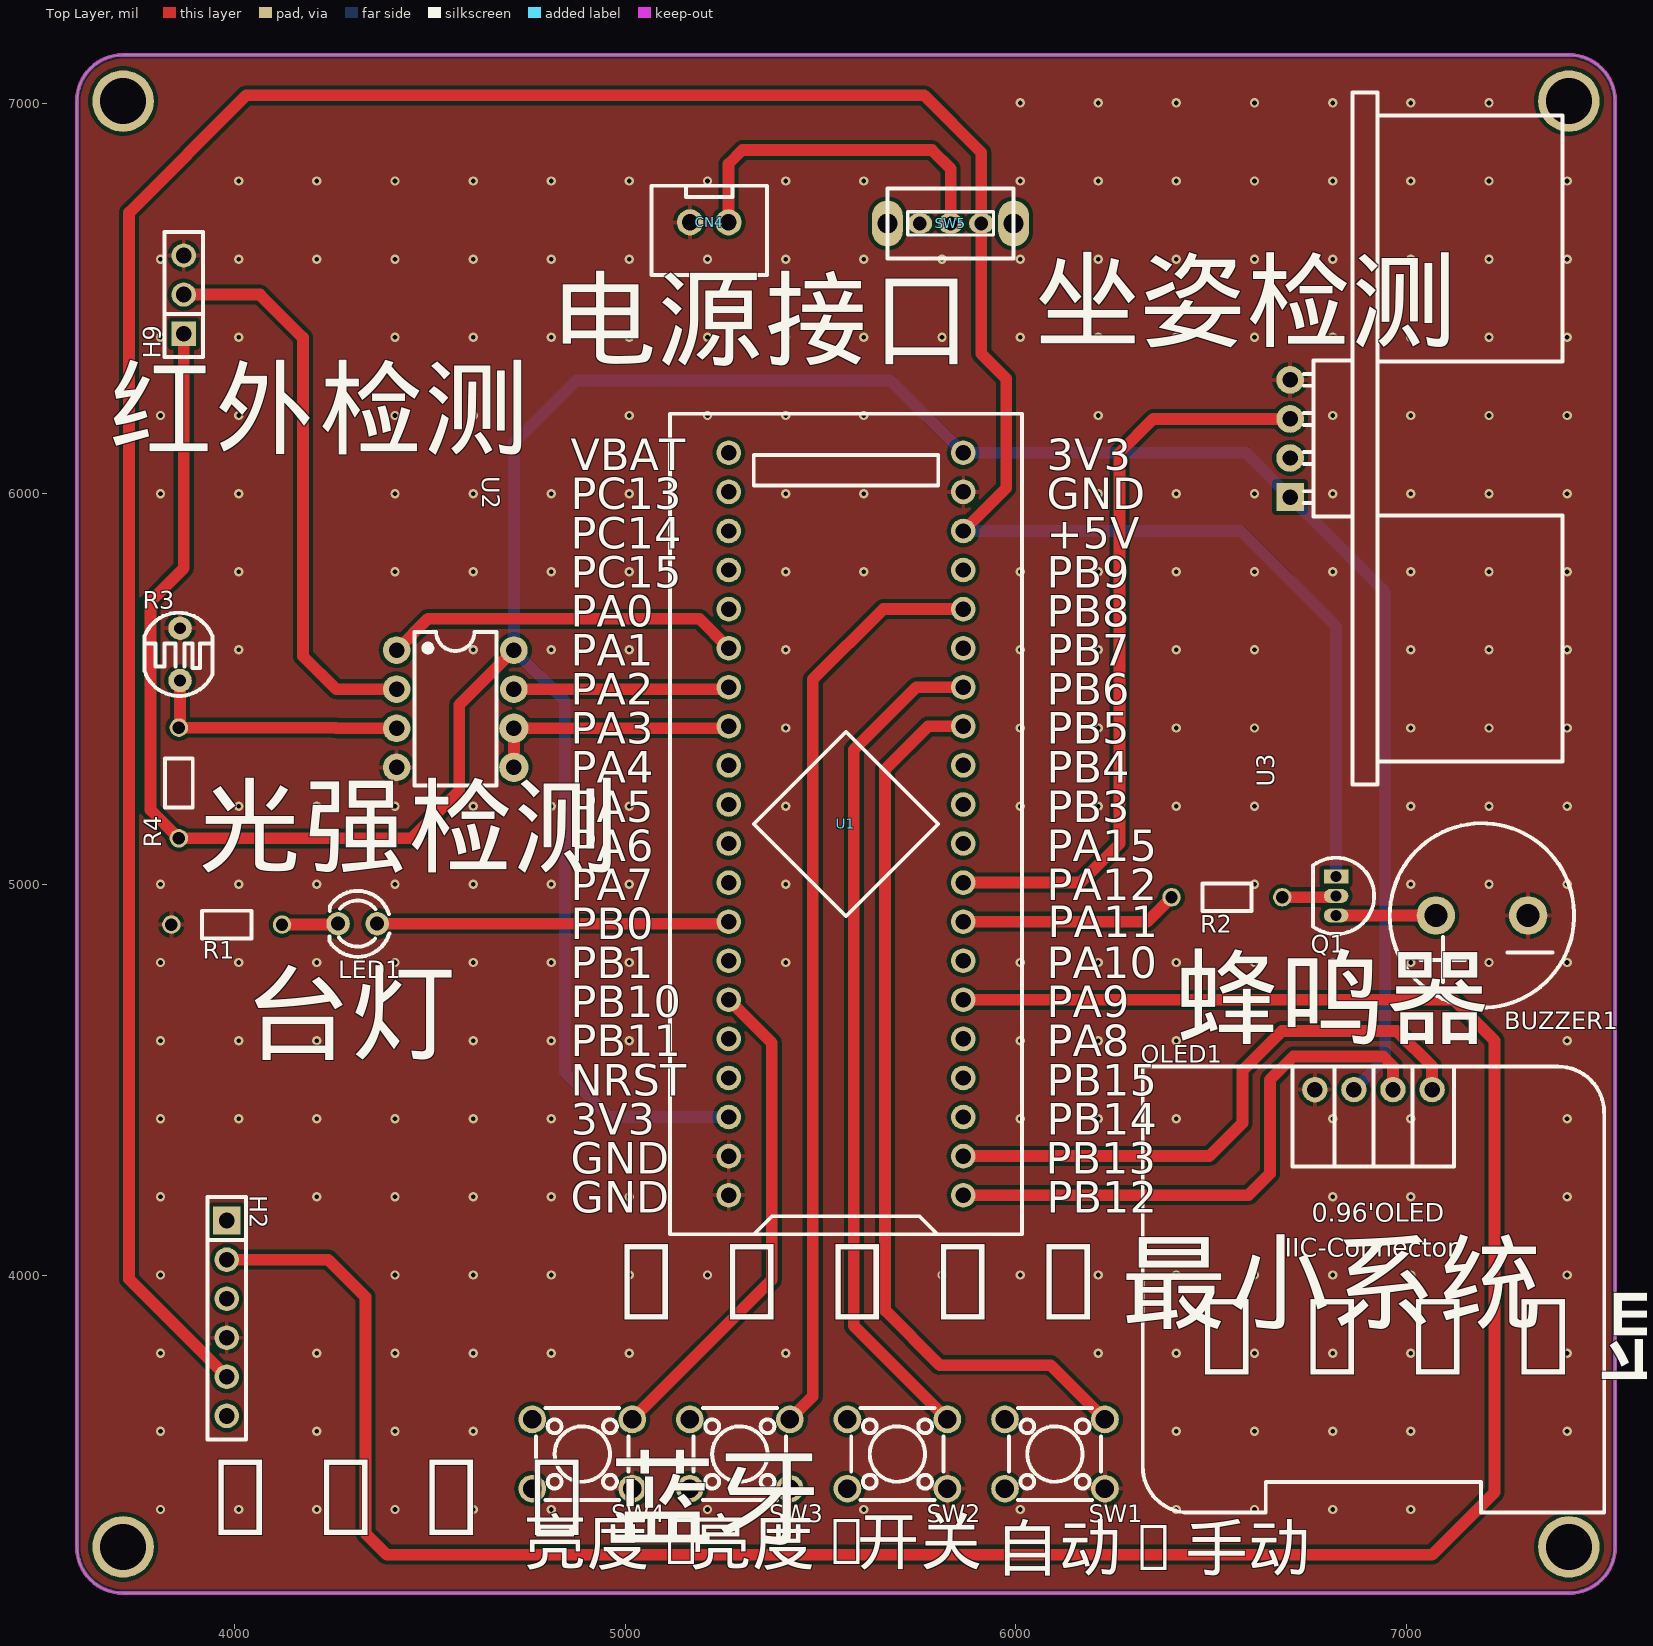
[diagram p0: Top Layer view]
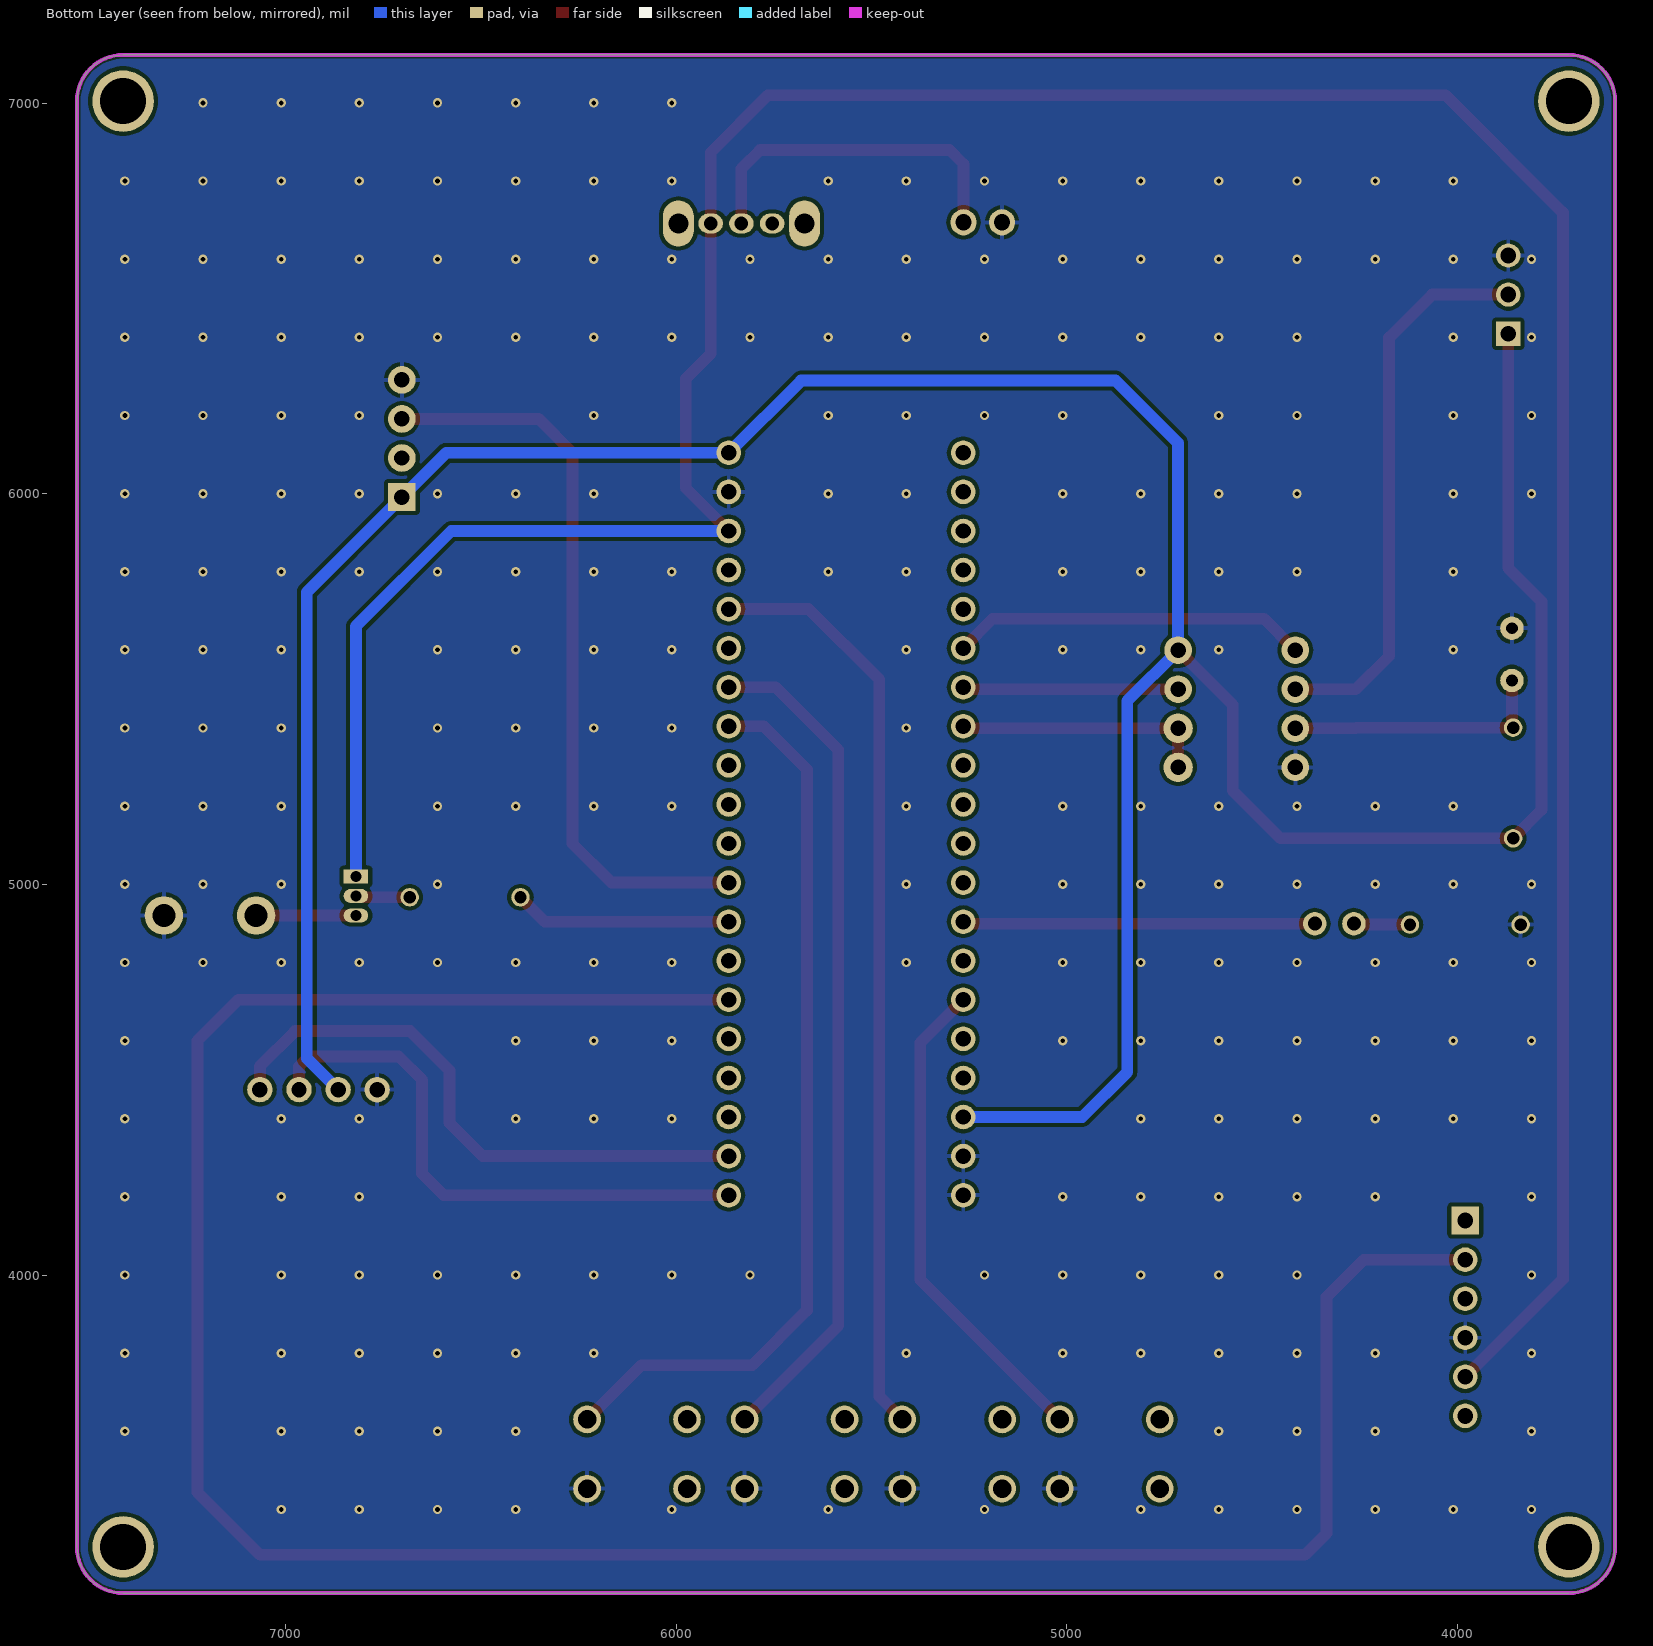
[diagram p1: Bottom Layer view, seen from below]
# Altium PCB MISC51796.pcbdoc
Units mil, origin at the board's own origin, x right, y up, seen from the top; angles counter-clockwise.
Board outline 3937.01 x 3937.01 mil, 2 copper layers (Top Layer, Bottom Layer), stack 62.206 mil thick; 19 components, 44 nets, 107 pads, 247 vias.

## Layer stack, top to bottom
Top Solder Mask Layer: solder mask 0.394, Dk 3.3
Top Layer: signal copper 1.379
Dielectric1: surface 59.449, FR4, Dk 4.5
Bottom Layer: signal copper 1.378
Bottom Solder Mask Layer: solder mask 0.394, Dk 3.3

## Board outline
3714.61,7123.5 ccw(c3714.61,7005.39) 3596.5,7005.39 3596.5,3304.61 ccw(c3714.61,3304.61) 3714.61,3186.5 7415.39,3186.5 ccw(c7415.39,3304.61) 7533.5,3304.61 7533.5,7005.39 ccw(c7415.39,7005.39) 7415.39,7123.5 3714.61,7123.5

## Design rules (kind name [scope] priority, off if disabled: settings)
BoardOutlineClearance copperThickness2oz_1 [All] p2 off: genericclearance=7.99 ignorepadtopadclearanceinfootprint=FALSE except(0: Arc-SplitContinuation Track-SplitContinuation SMDPad-SplitContinuation THPad-SplitContinuation Via-SplitContinuation Fill-SplitContinuation Region-SplitContinuation Poly-SplitContinuation Text-SplitContinuation Hole-SplitContinuation; 5.98: Arc-CutoutEdge Track-CutoutEdge SMDPad-CutoutEdge THPad-CutoutEdge Via-CutoutEdge Text-CutoutEdge; 6.9: Hole-OutlineEdge Hole-CutoutEdge; 10: Poly-OutlineEdge Poly-CutoutEdge; 11.81: Arc-OutlineEdge Track-OutlineEdge SMDPad-OutlineEdge THPad-OutlineEdge Via-OutlineEdge Fill-OutlineEdge Region-OutlineEdge Text-OutlineEdge Fill-CutoutEdge Region-CutoutEdge)
BoardOutlineClearance Plane_innerPlane_1 [All] p4 off: genericclearance=4.02 ignorepadtopadclearanceinfootprint=FALSE except(0: Arc-SplitContinuation Track-SplitContinuation SMDPad-SplitContinuation THPad-SplitContinuation Via-SplitContinuation Fill-SplitContinuation Region-SplitContinuation Poly-SplitContinuation Text-SplitContinuation Hole-SplitContinuation; 5.98: Arc-CutoutEdge Track-CutoutEdge SMDPad-CutoutEdge THPad-CutoutEdge Via-CutoutEdge Text-CutoutEdge; 6.9: Hole-OutlineEdge Hole-CutoutEdge; 10: Poly-OutlineEdge Poly-CutoutEdge; 11.81: Arc-OutlineEdge Track-OutlineEdge SMDPad-OutlineEdge THPad-OutlineEdge Via-OutlineEdge Fill-OutlineEdge Region-OutlineEdge Text-OutlineEdge Fill-CutoutEdge Region-CutoutEdge)
BoardOutlineClearance Copper_copperRegion_1 [All] p6 off: genericclearance=4.02 ignorepadtopadclearanceinfootprint=FALSE except(0: Arc-SplitContinuation Track-SplitContinuation SMDPad-SplitContinuation THPad-SplitContinuation Via-SplitContinuation Fill-SplitContinuation Region-SplitContinuation Poly-SplitContinuation Text-SplitContinuation Hole-SplitContinuation; 5.98: Arc-CutoutEdge Track-CutoutEdge SMDPad-CutoutEdge THPad-CutoutEdge Via-CutoutEdge Text-CutoutEdge; 6.9: Hole-OutlineEdge Hole-CutoutEdge; 10: Poly-OutlineEdge Poly-CutoutEdge; 11.81: Arc-OutlineEdge Track-OutlineEdge SMDPad-OutlineEdge THPad-OutlineEdge Via-OutlineEdge Fill-OutlineEdge Region-OutlineEdge Text-OutlineEdge Fill-CutoutEdge Region-CutoutEdge)
BoardOutlineClearance Copper_copperRegion_copperThickness1oz_1 [All] p8 off: genericclearance=4.02 ignorepadtopadclearanceinfootprint=FALSE except(0: Arc-SplitContinuation Track-SplitContinuation SMDPad-SplitContinuation THPad-SplitContinuation Via-SplitContinuation Fill-SplitContinuation Region-SplitContinuation Poly-SplitContinuation Text-SplitContinuation Hole-SplitContinuation; 5.98: Arc-CutoutEdge Track-CutoutEdge SMDPad-CutoutEdge THPad-CutoutEdge Via-CutoutEdge Text-CutoutEdge; 6.9: Hole-OutlineEdge Hole-CutoutEdge; 10: Poly-OutlineEdge Poly-CutoutEdge; 11.81: Arc-OutlineEdge Track-OutlineEdge SMDPad-OutlineEdge THPad-OutlineEdge Via-OutlineEdge Fill-OutlineEdge Region-OutlineEdge Text-OutlineEdge Fill-CutoutEdge Region-CutoutEdge)
BoardOutlineClearance Copper_copperRegion_Copper_copperRegion_1 [All] p10 off: genericclearance=4.02 ignorepadtopadclearanceinfootprint=FALSE except(0: Arc-SplitContinuation Track-SplitContinuation SMDPad-SplitContinuation THPad-SplitContinuation Via-SplitContinuation Fill-SplitContinuation Region-SplitContinuation Poly-SplitContinuation Text-SplitContinuation Hole-SplitContinuation; 5.98: Arc-CutoutEdge Track-CutoutEdge SMDPad-CutoutEdge THPad-CutoutEdge Via-CutoutEdge Text-CutoutEdge; 6.9: Hole-OutlineEdge Hole-CutoutEdge; 10: Poly-OutlineEdge Poly-CutoutEdge; 11.81: Arc-OutlineEdge Track-OutlineEdge SMDPad-OutlineEdge THPad-OutlineEdge Via-OutlineEdge Fill-OutlineEdge Region-OutlineEdge Text-OutlineEdge Fill-CutoutEdge Region-CutoutEdge)
BoardOutlineClearance copperThickness1oz_1 [All] p12: genericclearance=4.02 ignorepadtopadclearanceinfootprint=FALSE except(0: Arc-SplitContinuation Track-SplitContinuation SMDPad-SplitContinuation THPad-SplitContinuation Via-SplitContinuation Fill-SplitContinuation Region-SplitContinuation Poly-SplitContinuation Text-SplitContinuation Hole-SplitContinuation; 5.98: Arc-CutoutEdge Track-CutoutEdge SMDPad-CutoutEdge THPad-CutoutEdge Via-CutoutEdge Text-CutoutEdge; 6.9: Hole-OutlineEdge Hole-CutoutEdge; 10: Poly-OutlineEdge Poly-CutoutEdge; 11.81: Arc-OutlineEdge Track-OutlineEdge SMDPad-OutlineEdge THPad-OutlineEdge Via-OutlineEdge Fill-OutlineEdge Region-OutlineEdge Text-OutlineEdge Fill-CutoutEdge Region-CutoutEdge)
Clearance copperThickness2oz [All] p1 off: gap=7.99 ignorepadtopadclearanceinfootprint=FALSE except(5.98: SMDPad-Track SMDPad-SMDPad THPad-Track SMDPad-THPad THPad-THPad Track-Via SMDPad-Via THPad-Via Via-Via Fill-SMDPad Region-SMDPad Fill-THPad Region-THPad Fill-Via Region-Via Fill-Fill Fill-Region Region-Region Arc-Track Arc-SMDPad Arc-THPad Arc-Via Fill-Arc Region-Arc Arc-Arc Text-Track SMDPad-Text Text-THPad Text-Via Fill-Text Region-Text Arc-Text Text-Text; 6.9: Hole-Track Hole-SMDPad Hole-THPad Hole-Via Fill-Hole Region-Hole Hole-Arc Hole-Text; 10: Poly-Track Poly-SMDPad Poly-THPad Poly-Via Poly-Fill Poly-Region Poly-Poly Poly-Arc Poly-Text Poly-Hole; 11.81: Fill-Track Region-Track)
Clearance Plane_innerPlane [All] p3 off: gap=4.02 ignorepadtopadclearanceinfootprint=FALSE except(5.98: SMDPad-Track SMDPad-SMDPad THPad-Track SMDPad-THPad THPad-THPad Track-Via SMDPad-Via THPad-Via Via-Via Fill-SMDPad Region-SMDPad Fill-THPad Region-THPad Fill-Via Region-Via Fill-Fill Fill-Region Region-Region Arc-Track Arc-SMDPad Arc-THPad Arc-Via Fill-Arc Region-Arc Arc-Arc Text-Track SMDPad-Text Text-THPad Text-Via Fill-Text Region-Text Arc-Text Text-Text; 6.9: Hole-Track Hole-SMDPad Hole-THPad Hole-Via Fill-Hole Region-Hole Hole-Arc Hole-Text; 10: Poly-Track Poly-SMDPad Poly-THPad Poly-Via Poly-Fill Poly-Region Poly-Poly Poly-Arc Poly-Text Poly-Hole; 11.81: Fill-Track Region-Track)
Clearance Copper_copperRegion [All] p5 off: gap=4.02 ignorepadtopadclearanceinfootprint=FALSE except(5.98: SMDPad-Track SMDPad-SMDPad THPad-Track SMDPad-THPad THPad-THPad Track-Via SMDPad-Via THPad-Via Via-Via Fill-SMDPad Region-SMDPad Fill-THPad Region-THPad Fill-Via Region-Via Fill-Fill Fill-Region Region-Region Arc-Track Arc-SMDPad Arc-THPad Arc-Via Fill-Arc Region-Arc Arc-Arc Text-Track SMDPad-Text Text-THPad Text-Via Fill-Text Region-Text Arc-Text Text-Text; 6.9: Hole-Track Hole-SMDPad Hole-THPad Hole-Via Fill-Hole Region-Hole Hole-Arc Hole-Text; 10: Poly-Track Poly-SMDPad Poly-THPad Poly-Via Poly-Fill Poly-Region Poly-Poly Poly-Arc Poly-Text Poly-Hole; 11.81: Fill-Track Region-Track)
Clearance Copper_copperRegion_copperThickness1oz [All] p7 off: gap=4.02 ignorepadtopadclearanceinfootprint=FALSE except(5.98: SMDPad-Track SMDPad-SMDPad THPad-Track SMDPad-THPad THPad-THPad Track-Via SMDPad-Via THPad-Via Via-Via Fill-SMDPad Region-SMDPad Fill-THPad Region-THPad Fill-Via Region-Via Fill-Fill Fill-Region Region-Region Arc-Track Arc-SMDPad Arc-THPad Arc-Via Fill-Arc Region-Arc Arc-Arc Text-Track SMDPad-Text Text-THPad Text-Via Fill-Text Region-Text Arc-Text Text-Text; 6.9: Hole-Track Hole-SMDPad Hole-THPad Hole-Via Fill-Hole Region-Hole Hole-Arc Hole-Text; 10: Poly-Track Poly-SMDPad Poly-THPad Poly-Via Poly-Fill Poly-Region Poly-Poly Poly-Arc Poly-Text Poly-Hole; 11.81: Fill-Track Region-Track)
Clearance Copper_copperRegion_Copper_copperRegion [All] p9 off: gap=4.02 ignorepadtopadclearanceinfootprint=FALSE except(5.98: SMDPad-Track SMDPad-SMDPad THPad-Track SMDPad-THPad THPad-THPad Track-Via SMDPad-Via THPad-Via Via-Via Fill-SMDPad Region-SMDPad Fill-THPad Region-THPad Fill-Via Region-Via Fill-Fill Fill-Region Region-Region Arc-Track Arc-SMDPad Arc-THPad Arc-Via Fill-Arc Region-Arc Arc-Arc Text-Track SMDPad-Text Text-THPad Text-Via Fill-Text Region-Text Arc-Text Text-Text; 6.9: Hole-Track Hole-SMDPad Hole-THPad Hole-Via Fill-Hole Region-Hole Hole-Arc Hole-Text; 10: Poly-Track Poly-SMDPad Poly-THPad Poly-Via Poly-Fill Poly-Region Poly-Poly Poly-Arc Poly-Text Poly-Hole; 11.81: Fill-Track Region-Track)
Clearance copperThickness1oz [All] p11: gap=4.02 ignorepadtopadclearanceinfootprint=FALSE except(5.98: SMDPad-Track SMDPad-SMDPad THPad-Track SMDPad-THPad THPad-THPad Track-Via SMDPad-Via THPad-Via Via-Via Fill-SMDPad Region-SMDPad Fill-THPad Region-THPad Fill-Via Region-Via Fill-Fill Fill-Region Region-Region Arc-Track Arc-SMDPad Arc-THPad Arc-Via Fill-Arc Region-Arc Arc-Arc Text-Track SMDPad-Text Text-THPad Text-Via Fill-Text Region-Text Arc-Text Text-Text; 6.9: Hole-Track Hole-SMDPad Hole-THPad Hole-Via Fill-Hole Region-Hole Hole-Arc Hole-Text; 10: Poly-Track Poly-SMDPad Poly-THPad Poly-Via Poly-Fill Poly-Region Poly-Poly Poly-Arc Poly-Text Poly-Hole; 11.81: Fill-Track Region-Track)
DiffPairsRouting differentialPair [All] p1: maxlimit=6 minlimit=6 mostfreqgap=6 toplayer_minwidth=5 toplayer_prefwidth=10 toplayer_maxwidth=100 toplayer_mingap=6 toplayer_prefgap=6 toplayer_maxgap=6 bottomlayer_minwidth=5 bottomlayer_prefwidth=10 bottomlayer_maxwidth=100 bottomlayer_mingap=6 bottomlayer_prefgap=6 bottomlayer_maxgap=6 maxuncoupledlength=10
HoleToHoleClearance otherClearance [All] p1: gap=11.81 allowstackedmicrovias=TRUE
Length netLength [All] p1: minlimit=0 maxlimit=0
PasteMaskExpansion pasteMaskExpansion [All] p1: expansion=0
PlaneConnect innerPlane [All] p1: planeconnectstyle=Relief reliefexpansion=20 reliefentries=4 reliefconductorwidth=10 reliefairgap=10
PolygonConnect copperRegion_copperThickness1oz [All] p1 off: connectstyle=Relief reliefconductorwidth=10 reliefentries=4 polygonreliefangle="90 Angle" airgapwidth=10 via.connectstyle=Relief via.reliefconductorwidth=10 via.reliefentries=4 via.polygonreliefangle="90 Angle" via.airgapwidth=10
PolygonConnect copperRegion_Copper_copperRegion [All] p2 off: connectstyle=Relief reliefconductorwidth=10 reliefentries=4 polygonreliefangle="90 Angle" airgapwidth=10 via.connectstyle=Relief via.reliefconductorwidth=10 via.reliefentries=4 via.polygonreliefangle="90 Angle" via.airgapwidth=10
PolygonConnect copperRegion [All] p3: connectstyle=Relief reliefconductorwidth=10 reliefentries=4 polygonreliefangle="90 Angle" airgapwidth=10 via.connectstyle=Relief via.reliefconductorwidth=10 via.reliefentries=4 via.polygonreliefangle="90 Angle" via.airgapwidth=10
RoutingVias viaSize [All] p1: holewidth=12.01 width=24.02 viastyle="Through Hole" minholewidth=11.81 minwidth=19.68 maxholewidth=248.03 maxwidth=393.7
SolderMaskExpansion solderMaskExpansion [IsVia] p1: expansion=-1000 istentingtop=TRUE
SolderMaskExpansion solderMaskExpansion [All] p2: expansion=2 istentingtop=FALSE
Width copperThickness2oz_2 [All] p1 off: maxlimit=100 minlimit=8 preferedwidth=10
Width copperThickness1oz_2 [All] p2: maxlimit=100 minlimit=5 preferedwidth=10

## Components (designator, comment, footprint, x,y, rotation, side; value= is the part's Value field where it differs from the comment)
BUZZER1 "buzzer" BUZ-TH_BD12.0-P6.00-D0.9-RD 7192.78,4920.87 r180 top
CN4 "XH2.54*2P_直插" CONN-TH_2P-P2.50-XH2.54-2P 5215,6695 r0 top
H2 "" HDR-TH_6P-P2.54-V-F 3980,3890 r270 top
H9 "" HDR-TH_3P-P2.54-V-F 3870,6510 r90 top
LED1 "" LED_TH-3mm 4314.99,4899.94 r180 top
OLED1 "" 0.96OLED_4P 6915,4475 r0 top
Q1 "" S8550P_TO-92 6819.29,4970.87 r270 top
R1 "100" Res_1/8W 3980,4900 r180 top
R2 "1kΩ" Res_1/8W 6540,4970 r180 top
R3 "GL5549(80-100)" RES-TH_L5.1-W4.3-P3.40-D0.5 3860.5,5589.21 r0 top
R4 "10kΩ" Res_1/8W 3860,5260 r90 top
SW1 "" SW-TH_4P-L6.0-W6.0-P4.50-LS6.5 6099.85,3542.47 r180 top
SW2 "" SW-TH_4P-L6.0-W6.0-P4.50-LS6.5 5696.57,3542.47 r180 top
SW3 "" SW-TH_4P-L6.0-W6.0-P4.50-LS6.5 5293.28,3542.47 r180 top
SW4 "" SW-TH_4P-L6.0-W6.0-P4.50-LS6.5 4890,3542.47 r180 top
SW5 "" 拨动开关 5837.9,6692.05 r180 top
U1 "STM32F103C8T6-Card" CONN-TH_L53.3-W22.9_STM32F103C8T6-CARD 5565,5155 r90 top
U2 "ADC0832BCN" PDIP-8_L9.6-W6.4-P2.54-LS7.6-BL 4565,5450 r270 top
U3 "HC-SR04" TH_HC-SR04V 6701.72,6141.72 r90 top

## Footprints (in the part's own frame and the unit in brackets; to place one, negate y for a bottom-side part, rotate by r counter-clockwise, add the part's x,y. Pads: shape width x height; smd on the part's side, far side on the other; paste and mask are expansions set on the pad)
0.96OLED_4P [mm]
  round 1.65 hole 1 copper offset 0,0: 1(-3.81,-0.001) 2(-1.27,0.002) 3(1.27,0.002) 4(3.81,0.002)
  silkscreen extent -15,-27.5 15,1.5
BUZ-TH_BD12.0-P6.00-D0.9-RD [mm]
  round 2.5 hole 1.5 paste+0 mask+0.05: 1(-3,0) 2(3,0)
  silkscreen extent -5.99,-5.99 5.99,5.99
CONN-TH_2P-P2.50-XH2.54-2P [mm]
  round 1.7 hole 1.05 paste+0 mask+0.05: 1(1.25,0) 2(-1.25,0)
  silkscreen extent -3.75,-3.42 3.75,2.37
CONN-TH_L53.3-W22.9_STM32F103C8T6-CARD [mm]
  round 1.6 hole 1: 1(-24.13,-7.62) 2(-21.59,-7.62) 3(-19.05,-7.62) 4(-16.51,-7.62) 5(-13.97,-7.62) 6(-11.43,-7.62) 7(-8.89,-7.62) 8(-6.35,-7.62) 9(-3.81,-7.62) 10(-1.27,-7.62) 11(1.27,-7.62) 12(3.81,-7.62) 13(6.35,-7.62) 14(8.89,-7.62) 15(11.43,-7.62) 16(13.97,-7.62) 17(16.51,-7.62) 18(19.05,-7.62) 19(21.59,-7.62) 20(24.13,-7.62) 21(24.13,7.62) 22(21.59,7.62) 23(19.05,7.62) 24(16.51,7.62) 25(13.97,7.62) 26(11.43,7.62) 27(8.89,7.62) 28(6.35,7.62) 29(3.81,7.62) 30(1.27,7.62) 31(-1.27,7.62) 32(-3.81,7.62) 33(-6.35,7.62) 34(-8.89,7.62) 35(-11.43,7.62) 36(-13.97,7.62) 37(-16.51,7.62) 38(-19.05,7.62) 39(-21.59,7.62) 40(-24.13,7.62)
  silkscreen extent -26.67,-11.43 26.67,11.43
HDR-TH_3P-P2.54-V-F [mil]
  rect 62x62 hole 40.16: 1(-100,0)
  round 62 hole 40.16: 2(0,0) 3(100,0)
  silkscreen extent -160,-49 160,49
HDR-TH_6P-P2.54-V-F [mm]
  rect 1.8x1.8 hole 1.02: 1(-6.35,0)
  round 1.6 hole 1.02: 2(-3.81,0) 3(-1.27,0) 4(1.27,0) 5(3.81,0) 6(6.35,0)
  silkscreen extent -7.87,-1.25 7.87,1.25
LED_TH-3mm [mil]
  round 60 hole 36 paste+0 mask+2: 1(-50,0) 2(50,0)
  silkscreen extent -81,-84 72,85
PDIP-8_L9.6-W6.4-P2.54-LS7.6-BL [mm]
  round 1.8 hole 1: 1(-3.81,-3.81) 2(-1.27,-3.81) 3(1.27,-3.81) 4(3.81,-3.81) 7(-1.27,3.81) 8(-3.81,3.81)
  round 1.905 hole 1: 5(3.81,3.81) 6(1.27,3.81)
  silkscreen extent -5,-2.64 5,2.67
RES-TH_L5.1-W4.3-P3.40-D0.5 [mil]
  round 60 hole 30: 1(0,66.93) 2(0,-66.93)
  silkscreen extent -91,-106 83,106
Res_1/8W [mil]
  round 47.2 hole 31.5 paste+0 mask+2: 1(-141.7,2.48) 2(141.7,2.48)
  silkscreen extent -63,-33 63,38
S8550P_TO-92 [mm]
  rect 0.9x1.6 hole 0.7 paste+0 mask+0.051: 1(-1.27,0)
  oval 0.9x1.6 hole 0.7 paste+0 mask+0.051: 2(0,0) 3(1.27,0)
  silkscreen extent -2.48,-1.5 2.48,2.48
SW-TH_4P-L6.0-W6.0-P4.50-LS6.5 [mm]
  round 1.8 hole 1.2: 1(-3.25,2.25) 2(3.25,2.25) 3(-3.25,-2.25) 4(3.25,-2.25)
  silkscreen extent -3,-3 3,3
TH_HC-SR04V [mm]
  rect 1.8x1.8 hole 1.001: 1(-3.81,0)
  round 1.8 hole 1.001: 2(-1.27,0) 3(1.27,0) 4(3.81,0)
  silkscreen extent -22.5,-17.7 22.5,-0.89
拨动开关 [mil]
  oval 63x51.2 hole 35.4 paste+0 mask+2: 1(-73.4,0) 2(5,0) 3(84,0)
  oval 78.7x118.1 hole 51.2 paste+0 mask+2: 4(166.7,0) 5(-156.1,0)
  silkscreen extent -156,-90 167,90

## Free pads (board coordinates)
  round 157.48 hole 118.11: 1(3714.61,7005.39) 1(3714.61,3304.61) 1(7415.39,7005.39) 1(7415.39,3304.61)

## Via types
v1: diameter 24.02, hole 12, Top Layer to Bottom Layer, 247 vias

## Nets (pads, with @x,y where several pads share a name; then routed paths per layer and width w, separated by ;. In a path a pad name is that pad's centre, name@x,y a point inside that pad or via, vN(x,y) a via of type N, cw(c..) or ccw(c..) an arc to the next point about the centre after c; other vN are vias at no path point)
$1N17118: CN4.1 SW5.2 | length 892.6
  Top Layer w30: CN4.1 5264.22,6844.22 5300,6880 5785,6880 5832.9,6832.1 SW5.2
$1N17160: LED1.2 R1.1 | length 144.3
  Top Layer w30: R1.1 4262.57,4897.52 LED1.2
$1N17185: BUZZER1.2 Q1.3 | length 255.4
  Top Layer w30: Q1.3 BUZZER1.2
$1N17199: Q1.2 R2.1 | length 139
  Top Layer w30: R2.1 6815.95,4967.52 Q1.2
+5V: H2.5 Q1.1 SW5.1 U1.18 | length 8185.7
  Top Layer w30: H2.5 3730,3990 3730,6720 4030,7020 5765,7020 5911.3,6873.7 SW5.1 5911.3,6358.7 5975,6295 5975,6015 U1.18
  Bottom Layer w30: U1.18 6575,5905 6819.29,5660.71 Q1.1
CH0: H9.2 U2.2 | length 1440.8
  Top Layer w30: H9.2 4065,6510 4175,6400 4175,5585 4260,5500 U2.2
CH1: R3.2 R4.2 U2.3 | length 680
  Top Layer w30: R3.2 3860.5,5404.68 R4.2 4258.3,5401.7 4260,5400 U2.3
GND: BUZZER1.1 CN4.2 H2.4 H9.3 OLED1.1 R1.2 R3.1 SW1.1 SW2.1 SW3.1 SW4.1 U1.19 U1.39 U1.40 U2.4 U3.4
  other v1: 3810.6,3400.6 4010.6,3400.6 4210.6,3400.6 4410.6,3400.6 4610.6,3400.6 4810.6,3400.6 5210.6,3400.6 5610.6,3400.6 6010.6,3400.6 6410.6,3400.6 6610.6,3400.6 6810.6,3400.6 7010.6,3400.6 3810.6,3600.6 4210.6,3600.6 4410.6,3600.6 4610.6,3600.6 6410.6,3600.6 6610.6,3600.6 6810.6,3600.6 7010.6,3600.6 7410.6,3600.6 3810.6,3800.6 4210.6,3800.6 4410.6,3800.6 4610.6,3800.6 4810.6,3800.6 5010.6,3800.6 5410.6,3800.6 6210.6,3800.6 6410.6,3800.6 6610.6,3800.6 6810.6,3800.6 7010.6,3800.6 7410.6,3800.6 3810.6,4000.6 4410.6,4000.6 4610.6,4000.6 4810.6,4000.6 5010.6,4000.6 5210.6,4000.6 5810.6,4000.6 6010.6,4000.6 6210.6,4000.6 6410.6,4000.6 6610.6,4000.6 6810.6,4000.6 7010.6,4000.6 7410.6,4000.6 3810.6,4200.6 4210.6,4200.6 4410.6,4200.6 4610.6,4200.6 4810.6,4200.6 5010.6,4200.6 6810.6,4200.6 7010.6,4200.6 7410.6,4200.6 3810.6,4400.6 4010.6,4400.6 4210.6,4400.6 4410.6,4400.6 4610.6,4400.6 4810.6,4400.6 6010.6,4400.6 6210.6,4400.6 6410.6,4400.6 6810.6,4400.6 7010.6,4400.6 7410.6,4400.6 3810.6,4600.6 4010.6,4600.6 4210.6,4600.6 4410.6,4600.6 4610.6,4600.6 4810.6,4600.6 5010.6,4600.6 6010.6,4600.6 6210.6,4600.6 6410.6,4600.6 7410.6,4600.6 3810.6,4800.6 4010.6,4800.6 4210.6,4800.6 4410.6,4800.6 4610.6,4800.6 4810.6,4800.6 5010.6,4800.6 5410.6,4800.6 6010.6,4800.6 6210.6,4800.6 6410.6,4800.6 6610.6,4800.6 6810.6,4800.6 7010.6,4800.6 7210.6,4800.6 7410.6,4800.6 3810.6,5000.6 4010.6,5000.6 4210.6,5000.6 4410.6,5000.6 4610.6,5000.6 4810.6,5000.6 5010.6,5000.6 5410.6,5000.6 6610.6,5000.6 7010.6,5000.6 7210.6,5000.6 7410.6,5000.6 4010.6,5200.6 4210.6,5200.6 4410.6,5200.6 4610.6,5200.6 4810.6,5200.6 5010.6,5200.6 5410.6,5200.6 6010.6,5200.6 6210.6,5200.6 6410.6,5200.6 6610.6,5200.6 7010.6,5200.6 7210.6,5200.6 7410.6,5200.6 5410.6,5400.6 6010.6,5400.6 6210.6,5400.6 6410.6,5400.6 6610.6,5400.6 7010.6,5400.6 7210.6,5400.6 7410.6,5400.6 4010.6,5600.6 4610.6,5600.6 4810.6,5600.6 5010.6,5600.6 5410.6,5600.6 6010.6,5600.6 6210.6,5600.6 6410.6,5600.6 6610.6,5600.6 7010.6,5600.6 7210.6,5600.6 7410.6,5600.6 4010.6,5800.6 4410.6,5800.6 4610.6,5800.6 4810.6,5800.6 5010.6,5800.6 5410.6,5800.6 5610.6,5800.6 6010.6,5800.6 6210.6,5800.6 6410.6,5800.6 6610.6,5800.6 6810.6,5800.6 7010.6,5800.6 7210.6,5800.6 7410.6,5800.6 3810.6,6000.6 4010.6,6000.6 4410.6,6000.6 4610.6,6000.6 4810.6,6000.6 5010.6,6000.6 5410.6,6000.6 5610.6,6000.6 6210.6,6000.6 6410.6,6000.6 6610.6,6000.6 6810.6,6000.6 7010.6,6000.6 7210.6,6000.6 7410.6,6000.6 3810.6,6200.6 4010.6,6200.6 4410.6,6200.6 4610.6,6200.6 5010.6,6200.6 5210.6,6200.6 5410.6,6200.6 5610.6,6200.6 6210.6,6200.6 6810.6,6200.6 7010.6,6200.6 7210.6,6200.6 7410.6,6200.6 3810.6,6400.6 4010.6,6400.6 4410.6,6400.6 4610.6,6400.6 4810.6,6400.6 5010.6,6400.6 5210.6,6400.6 5410.6,6400.6 5610.6,6400.6 5810.6,6400.6 6010.6,6400.6 6210.6,6400.6 6410.6,6400.6 6610.6,6400.6 6810.6,6400.6 7010.6,6400.6 7210.6,6400.6 7410.6,6400.6 3810.6,6600.6 4010.6,6600.6 4210.6,6600.6 4410.6,6600.6 4610.6,6600.6 4810.6,6600.6 5010.6,6600.6 5210.6,6600.6 5410.6,6600.6 5610.6,6600.6 5810.6,6600.6 6010.6,6600.6 6210.6,6600.6 6410.6,6600.6 6610.6,6600.6 6810.6,6600.6 7010.6,6600.6 7210.6,6600.6 7410.6,6600.6 4010.6,6800.6 4210.6,6800.6 4410.6,6800.6 4610.6,6800.6 4810.6,6800.6 5010.6,6800.6 5210.6,6800.6 5410.6,6800.6 5610.6,6800.6 6010.6,6800.6 6210.6,6800.6 6410.6,6800.6 6610.6,6800.6 6810.6,6800.6 7010.6,6800.6 7210.6,6800.6 7410.6,6800.6 6010.6,7000.6 6210.6,7000.6 6410.6,7000.6 6610.6,7000.6 6810.6,7000.6 7010.6,7000.6 7210.6,7000.6
NRST: U1.37
PA0: U1.25
PA1: U1.26 U2.1 | length 914.2
  Top Layer w30: U2.1 4495,5680 5190,5680 U1.26
PA2: U1.27 U2.7 | length 552.1
  Top Layer w30: U2.7 5260,5500 U1.27
PA3: U1.28 U2.5 U2.6 | length 662.1
  Top Layer w30: U2.5@4715,5290 U2.6 5260,5400 U1.28
PA4: U1.29
PA5: U1.30
PA6: U1.31
PA7: U1.32
PA8: U1.5
PA9: H2.2 U1.6 | length 6536.9
  Top Layer w30: H2.2 4240,4040 4335,3945 4335,3340 4390,3285 7065,3285 7225,3445 7225,4600 7120,4705 U1.6
PA10: U1.7
PA11: R2.2 U1.8 | length 559.2
  Top Layer w30: U1.8 6335.78,4905 R2.2
PA12: U1.9 U3.3 | length 1914.1
  Top Layer w30: U1.9 6165,5005 6265,5105 6265,6105 6351.72,6191.72 U3.3
PA14: U3.2
PA15: U1.10
PB0: LED1.1 U1.33 | length 902.1
  Top Layer w30: LED1.1 5259.94,4899.94 U1.33
PB1: U1.34
PB3: U1.11
PB4: U1.12
PB5: SW1.3 U1.13 | length 2308.9
  Top Layer w30: U1.13 5775,5405 5665,5295 5665,3910 5805,3770 6088.85,3770 SW1.3
PB6: SW2.3 U1.14 | length 2159.4
  Top Layer w30: SW2.3 5585,3870.57 5585,5345 5745,5505 U1.14
PB7: U1.15
PB8: SW3.3 U1.16 | length 2377.9
  Top Layer w30: SW3.3 5480,3689.82 5480,5525 5660,5705 U1.16
PB9: U1.17
PB10: SW4.3 U1.35 | length 1267.4
  Top Layer w30: SW4.3 5375,3988.1 5375,4595 U1.35
PB11: U1.36
PB12: OLED1.3 U1.1 | length 1457.9
  Top Layer w30: U1.1 6595,4205 6650,4260 6650,4500 6710,4560 6940,4560 6965,4535 OLED1.3@6965,4475.05
PB13: OLED1.4 U1.2 | length 1508.9
  Top Layer w30: U1.2 6495,4305 6580,4390 6580,4525 6680,4625 6975,4625 7065,4535 OLED1.4@7065,4475.05
PB14: U1.3
PB15: U1.4
PC13: U1.22
PC14: U1.23
PC15: U1.24
VBAT: U1.21
VCC: H9.1 OLED1.2 R4.1 U1.20 U1.38 U2.8 U3.1 | length 8501.4
  Top Layer w30: H9.1 3870,5810 3785,5725 3785,5190.82 R4.1 4453.3,5118.3 4575,5240 4575,5460 U2.8
  Bottom Layer w30: U1.38 4960,4405 4845,4520 4845,5470 U2.8 4715,6130 4875,6290 5680,6290 U1.20 6588.43,6105 U3.1 6945,5748.43 6945,4555.05 OLED1.2@6865,4475.05
pads on no net: H2.1 H2.3 H2.6 SW1.2 SW1.4 SW2.2 SW2.4 SW3.2 SW3.4 SW4.2 SW4.4 SW5.3 SW5.4 SW5.5

## Polygon pours and split planes (outlines as drawn)
GND on Bottom Layer (solid, remove dead copper, pour order 2): 3525,7245 3525,3080 7700,3080 7700,7245
GND on Top Layer (solid, remove dead copper, pour order 2): 3000,7415 3000,3000 7930,3000 7930,7415

## Keep-outs
Board Outline Layer:
  the board outline again, w10

## Silkscreen, mask and mechanical layers (free items; w line width, h text height)
Top Silkscreen Layer:
  text "坐姿检测" at 6050,6400 h196.85
  text "电源接口" at 4812.87,6351.57 h196.85
  text "红外检测" at 3675,6125 h196.85
  text "VBAT" at 4860.95,6060 h80
  text "3V3" at 6079.16,6060 h80
  text "PC13" at 4860.95,5960 h80
  text "GND" at 6079.16,5960 h80
  text "PC14" at 4860.95,5860 h80
  text "+5V" at 6079.16,5860 h80
  text "PC15" at 4860.95,5760 h80
  text "PB9" at 6079.16,5760 h80
  text "PA0" at 4860.95,5660 h80
  text "PB8" at 6079.16,5660 h80
  text "PA1" at 4860.95,5560 h80
  text "PB7" at 6079.16,5560 h80
  text "PA2" at 4860.95,5460 h80
  text "PB6" at 6079.16,5460 h80
  text "PA3" at 4860.95,5360 h80
  text "PB5" at 6079.16,5360 h80
  text "PA4" at 4860.95,5260 h80
  text "PB4" at 6079.16,5260 h80
  text "PA5" at 4860.95,5160 h80
  text "PB3" at 6079.16,5160 h80
  text "PA6" at 4860.95,5060 h80
  text "PA15" at 6079.16,5060 h80
  text "光强检测" at 3905,5055 h196.85
  text "PA7" at 4860.95,4960 h80
  text "PA12" at 6079.16,4960 h80
  text "PA11" at 6080.95,4865 h80
  text "PB0" at 4860.95,4860 h80
  text "PB1" at 4860.95,4760 h80
  text "PA10" at 6079.16,4760 h80
  text "PB10" at 4860.95,4660 h80
  text "PA9" at 6079.16,4660 h80
  text "蜂鸣器" at 6405,4615 h196.85
  text "台灯" at 4030,4575 h196.85
  text "PB11" at 4860.95,4560 h80
  text "PA8" at 6079.16,4560 h80
  text "NRST" at 4860.95,4460 h80
  text "PB15" at 6079.16,4460 h80
  text "3V3" at 4860.95,4360 h80
  text "PB14" at 6079.16,4360 h80
  text "GND" at 4860.95,4260 h80
  text "PB13" at 6075.95,4260 h80
  text "GND" at 4860.95,4160 h80
  text "PB12" at 6079.16,4160 h80
  text "STM32最小系统" at 4919.45,3886.57 h196.85
  text "Oled显示器" at 6405,3745 h196.85
  text "HC05蓝牙" at 3880,3335 h196.85
  text "开关" at 5592.45,3262.15 h118.11
  text "亮度-" at 4740,3260 h118.11
  text "亮度+" at 5163.36,3260 h118.11
  text "自动/手动" at 5950,3245.15 h118.11